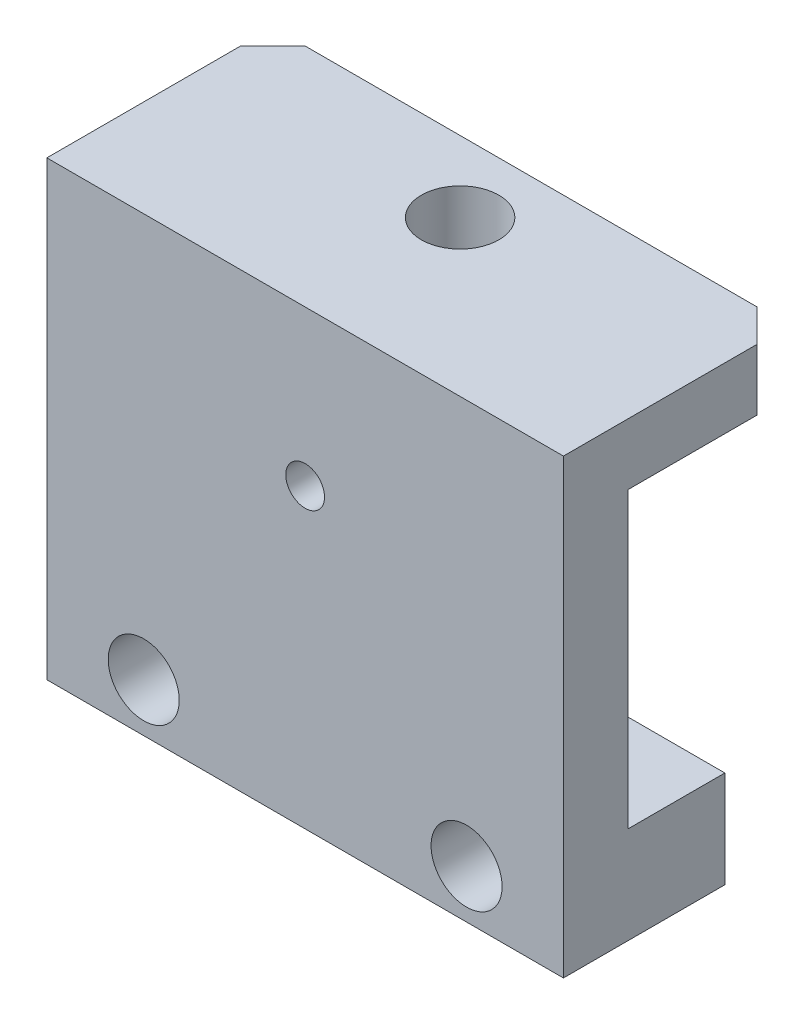
from build123d import *

# Parameters (mm, degrees)
SKETCH_1_W                   = 80
SKETCH_1_H                   = 70
EXTRUDE_1_DEPTH              = 25
SKETCH_2_W                   = 15
SKETCH_2_H                   = 45.5
CUT_EXTRUDE_1_DEPTH          = 109
HOLE_WIZARD_M6_1_D           = 6.4
HOLE_WIZARD_M6_1_CBORE_D     = 11
HOLE_WIZARD_M6_1_CBORE_DEPTH = 6.4
SKETCH_7_R                   = 5.5
CUT_EXTRUDE_3_DEPTH          = 10
SKETCH_8_R                   = 3
CUT_EXTRUDE_4_DEPTH          = 10
SKETCH_9_W                   = 80
SKETCH_9_H                   = 9.5
EXTRUDE_2_DEPTH              = 10
SKETCH_10_R                  = 6
CUT_EXTRUDE_5_DEPTH          = 9.5
CHAMFER_1_SIZE               = 5


with BuildPart() as part:
    # 草图1 → 凸台-拉伸1 (new body)
    with BuildSketch(Plane.XY):
        with Locations((40, 35)):
            Rectangle(SKETCH_1_W, SKETCH_1_H)
    extrude(amount=EXTRUDE_1_DEPTH)

    # 草图2 → 切除-拉伸1 (cut)
    with BuildSketch(Plane(origin=(80, 0, 0), x_dir=(0, 0, -1), z_dir=(1, 0, 0))):
        with Locations((-7.5, 37.75)):
            Rectangle(SKETCH_2_W, SKETCH_2_H)
    extrude(amount=-CUT_EXTRUDE_1_DEPTH, mode=Mode.SUBTRACT)

    # M6 六角凹头螺钉的柱形沉头孔1 (through all)
    with Locations(Plane.XY.offset(25)):
        with Locations((15, 7.5), (65, 7.5)):
            CounterBoreHole(HOLE_WIZARD_M6_1_D / 2, HOLE_WIZARD_M6_1_CBORE_D / 2, HOLE_WIZARD_M6_1_CBORE_DEPTH)

    # 草图7 → 切除-拉伸3 (cut)
    with BuildSketch(Plane.XY.offset(18.6)):
        with Locations((15, 7.5)):
            Circle(SKETCH_7_R)
        with Locations((65, 7.5)):
            Circle(SKETCH_7_R)
    extrude(amount=-CUT_EXTRUDE_3_DEPTH, mode=Mode.SUBTRACT)

    # 草图8 → 切除-拉伸4 (cut)
    with BuildSketch(Plane.XY.offset(25)):
        with Locations((40, 46)):
            Circle(SKETCH_8_R)
    extrude(amount=-CUT_EXTRUDE_4_DEPTH, mode=Mode.SUBTRACT)

    # 草图9 → 凸台-拉伸2 (add)
    with BuildSketch(Plane(origin=(0, 0, 0), x_dir=(-1, 0, 0), z_dir=(0, 0, -1))):
        with Locations((-40, 65.25)):
            Rectangle(SKETCH_9_W, SKETCH_9_H)
    extrude(amount=EXTRUDE_2_DEPTH)

    # 草图10 → 切除-拉伸5 (cut)
    with BuildSketch(Plane(origin=(0, 70, 0), x_dir=(1, 0, 0), z_dir=(0, 1, 0))):
        with Locations(Location((40, -1, 0), (0, 0, 270))):
            Circle(SKETCH_10_R)
    extrude(amount=-CUT_EXTRUDE_5_DEPTH, mode=Mode.SUBTRACT)

    # 倒角1
    chamfer_1_edges = [part.edges().sort_by_distance(p)[0] for p in [
        (80, 65.25, -10),
        (0, 65.25, -10),
    ]]
    chamfer(chamfer_1_edges, length=CHAMFER_1_SIZE)


solid = part.part
